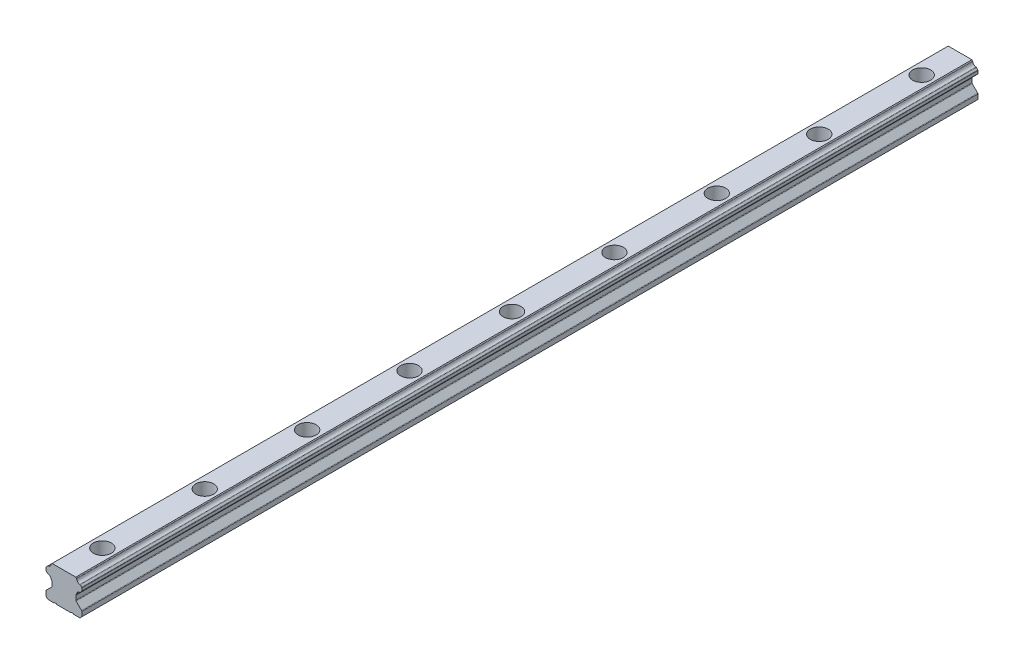
from build123d import *

# Parameters (mm, degrees)
EXTRUDE_1_DEPTH              = 700
CUT_EXTRUDE_1_DEPTH          = 701.622580281
CUT_EXTRUDE_2_REACH          = 702.623
SKETCH_4_W                   = 1.2
SKETCH_4_H                   = 0.5
CUT_EXTRUDE_3_DEPTH          = 701.622580281
SKETCH_5_W                   = 1.2
SKETCH_5_H                   = 0.5
CUT_EXTRUDE_4_DEPTH          = 701.622580281
CUT_EXTRUDE_5_DEPTH          = 701.622580281
CUT_EXTRUDE_6_REACH          = 702.623
CUT_EXTRUDE_7_REACH          = 702.623
CUT_EXTRUDE_8_REACH          = 702.623
DRAFT_1_ANGLE                = 45
DRAFT_2_ANGLE                = 45
DRAFT_3_ANGLE                = 45
DRAFT_4_ANGLE                = 45
HOLE_WIZARD_M8_1_D           = 9
HOLE_WIZARD_M8_1_CBORE_D     = 14
HOLE_WIZARD_M8_1_CBORE_DEPTH = 12
CHAMFER_1_SIZE               = 1.5
FILLET_1_R                   = 0.6
FILLET_2_R                   = 0.8


with BuildPart() as part:
    # 草图1 → 凸台-拉伸1 (new body)
    with BuildSketch(Plane(origin=(0, 0, -110), x_dir=(-1, 0, 0), z_dir=(0, 0, -1))):
        Polygon((-14, -4.744169479), (-14, -26), (14, -26), (14, -4.744169479), (9.255830521, 0), (-9.255830521, 0), align=None)
    extrude(amount=-EXTRUDE_1_DEPTH)

    # 草图2 → 切除-拉伸1 (cut, through all)
    with BuildSketch(Plane.XY.offset(590)):
        Polygon((14, -7.261680545), (9.3, -11.961680545), (9.3, -15.858900345), (14, -15.858900345), align=None)
    extrude(amount=-CUT_EXTRUDE_1_DEPTH, mode=Mode.SUBTRACT)

    # 草图3 → 切除-拉伸2 (cut, up to next)
    with BuildSketch(Plane.XY.offset(590), mode=Mode.PRIVATE) as cut_extrude_2_sk1:
        with BuildLine():
            Line((9.901074838, -11.360605707), (12.569687707, -8.691992838))
            ThreePointArc((12.569687707, -8.691992838), (10.725602827, -9.516520827), (9.901074838, -11.360605707))
        make_face()
    cut_extrude_2_tool1 = extrude(cut_extrude_2_sk1.sketch, amount=-CUT_EXTRUDE_2_REACH, mode=Mode.PRIVATE) & part.part
    add(cut_extrude_2_tool1.solids().sort_by_distance((11.029066, -9.819984, 590))[0], mode=Mode.SUBTRACT)

    # 草图4 → 切除-拉伸3 (cut, through all)
    with BuildSketch(Plane.XY.offset(590)):
        with Locations((6.65, -25.75)):
            Rectangle(SKETCH_4_W, SKETCH_4_H)
    extrude(amount=-CUT_EXTRUDE_3_DEPTH, mode=Mode.SUBTRACT)

    # 草图5 → 切除-拉伸4 (cut, through all)
    with BuildSketch(Plane.XY.offset(590)):
        with Locations((-6.65, -25.75)):
            Rectangle(SKETCH_5_W, SKETCH_5_H)
    extrude(amount=-CUT_EXTRUDE_4_DEPTH, mode=Mode.SUBTRACT)

    # 草图6 → 切除-拉伸5 (cut, through all)
    with BuildSketch(Plane.XY.offset(590)):
        Polygon((-14, -20.558900345), (-9.3, -20.558900345), (-9.3, -11.961680545), (-14, -7.261680545), align=None)
    extrude(amount=-CUT_EXTRUDE_5_DEPTH, mode=Mode.SUBTRACT)

    # 草图7 → 切除-拉伸6 (cut, up to next)
    with BuildSketch(Plane.XY.offset(590), mode=Mode.PRIVATE) as cut_extrude_6_sk1:
        with BuildLine():
            Line((-12.569687707, -8.691992838), (-9.901074838, -11.360605707))
            ThreePointArc((-9.901074838, -11.360605707), (-10.725602827, -9.516520827), (-12.569687707, -8.691992838))
        make_face()
    cut_extrude_6_tool1 = extrude(cut_extrude_6_sk1.sketch, amount=-CUT_EXTRUDE_6_REACH, mode=Mode.PRIVATE) & part.part
    add(cut_extrude_6_tool1.solids().sort_by_distance((-11.029066, -9.819984, 590))[0], mode=Mode.SUBTRACT)

    # 草图8 → 切除-拉伸7 (cut, up to next)
    with BuildSketch(Plane.XY.offset(590), mode=Mode.PRIVATE) as cut_extrude_7_sk1:
        with BuildLine():
            Line((-9.901411286, -0.645580765), (-12.563746235, -3.307915714))
            ThreePointArc((-12.563746235, -3.307915714), (-10.725602827, -2.483724173), (-9.901411286, -0.645580765))
        make_face()
    cut_extrude_7_tool1 = extrude(cut_extrude_7_sk1.sketch, amount=-CUT_EXTRUDE_7_REACH, mode=Mode.PRIVATE) & part.part
    add(cut_extrude_7_tool1.solids().sort_by_distance((-11.027412, -2.181915, 590))[0], mode=Mode.SUBTRACT)

    # 草图9 → 切除-拉伸8 (cut, up to next)
    with BuildSketch(Plane.XY.offset(590), mode=Mode.PRIVATE) as cut_extrude_8_sk1:
        with BuildLine():
            Line((12.563746235, -3.307915714), (9.901411286, -0.645580765))
            ThreePointArc((9.901411286, -0.645580765), (10.725602827, -2.483724173), (12.563746235, -3.307915714))
        make_face()
    cut_extrude_8_tool1 = extrude(cut_extrude_8_sk1.sketch, amount=-CUT_EXTRUDE_8_REACH, mode=Mode.PRIVATE) & part.part
    add(cut_extrude_8_tool1.solids().sort_by_distance((11.027412, -2.181915, 590))[0], mode=Mode.SUBTRACT)

    # 拔模1
    draft_1_faces = [part.faces().sort_by_distance(p)[0] for p in [
        (11.65, -15.858900345, 240),
    ]]
    draft(draft_1_faces, Plane(origin=(9.3, -11.961680545, -110), x_dir=(0, 0, 1), z_dir=(1, 0, 0)), DRAFT_1_ANGLE)

    # 拔模2
    draft_2_faces = [part.faces().sort_by_distance(p)[0] for p in [
        (-11.65, -20.558900345, 240),
    ]]
    draft(draft_2_faces, Plane(origin=(-14, -26, 590), x_dir=(0, 0, -1), z_dir=(-1, 0, 0)), DRAFT_2_ANGLE)

    # 拔模3
    draft_3_faces = [part.faces().sort_by_distance(p)[0] for p in [
        (6.05, -25.75, 240),
        (7.25, -25.75, 240),
    ]]
    draft(draft_3_faces, Plane(origin=(7.25, -25.5, -110), x_dir=(0, 0, -1), z_dir=(0, -1, 0)), DRAFT_3_ANGLE)

    # 拔模4
    draft_4_faces = [part.faces().sort_by_distance(p)[0] for p in [
        (-7.25, -25.75, 240),
        (-6.05, -25.75, 240),
    ]]
    draft(draft_4_faces, Plane(origin=(-6.05, -25.5, -110), x_dir=(0, 0, -1), z_dir=(0, -1, 0)), DRAFT_4_ANGLE)

    # M8 六角头螺栓的柱形沉头孔1 (through all)
    with Locations(Plane(origin=(0, 0, 0), x_dir=(1, 0, 0), z_dir=(0, 1, 0))):
        with Locations((0, -160), (0, -240), (0, -320), (0, -400), (0, -480), (0, -560), (0, 80), (0, -80), (0, 0)):
            CounterBoreHole(HOLE_WIZARD_M8_1_D / 2, HOLE_WIZARD_M8_1_CBORE_D / 2, HOLE_WIZARD_M8_1_CBORE_DEPTH)

    # 倒角1
    chamfer_1_edges = [part.edges().sort_by_distance(p)[0] for p in [
        (-14, -26, 240),
        (14, -26, 240),
    ]]
    chamfer(chamfer_1_edges, length=CHAMFER_1_SIZE)

    # 圆角1
    fillet_1_edges = [part.edges().sort_by_distance(p)[0] for p in [
        (-12.569687707, -8.691992838, 240),
        (-9.901074838, -11.360605707, 240),
        (-14, -4.744169479, 240),
        (14, -4.744169479, 240),
        (-9.901411286, -0.645580765, 240),
        (-12.563746235, -3.307915714, 240),
        (12.563746235, -3.307915714, 240),
        (9.901411286, -0.645580765, 240),
        (14, -7.261680545, 240),
        (9.901074838, -11.360605707, 240),
        (12.569687707, -8.691992838, 240),
        (-14, -7.261680545, 240),
    ]]
    fillet(fillet_1_edges, radius=FILLET_1_R)

    # 圆角2
    fillet_2_edges = [part.edges().sort_by_distance(p)[0] for p in [
        (14, -20.558900345, 240),
        (9.3, -15.858900345, 240),
        (9.3, -11.961680545, 240),
        (-14, -20.558900345, 240),
        (-9.3, -11.961680545, 240),
        (-9.3, -15.858900345, 240),
    ]]
    fillet(fillet_2_edges, radius=FILLET_2_R)


solid = part.part
